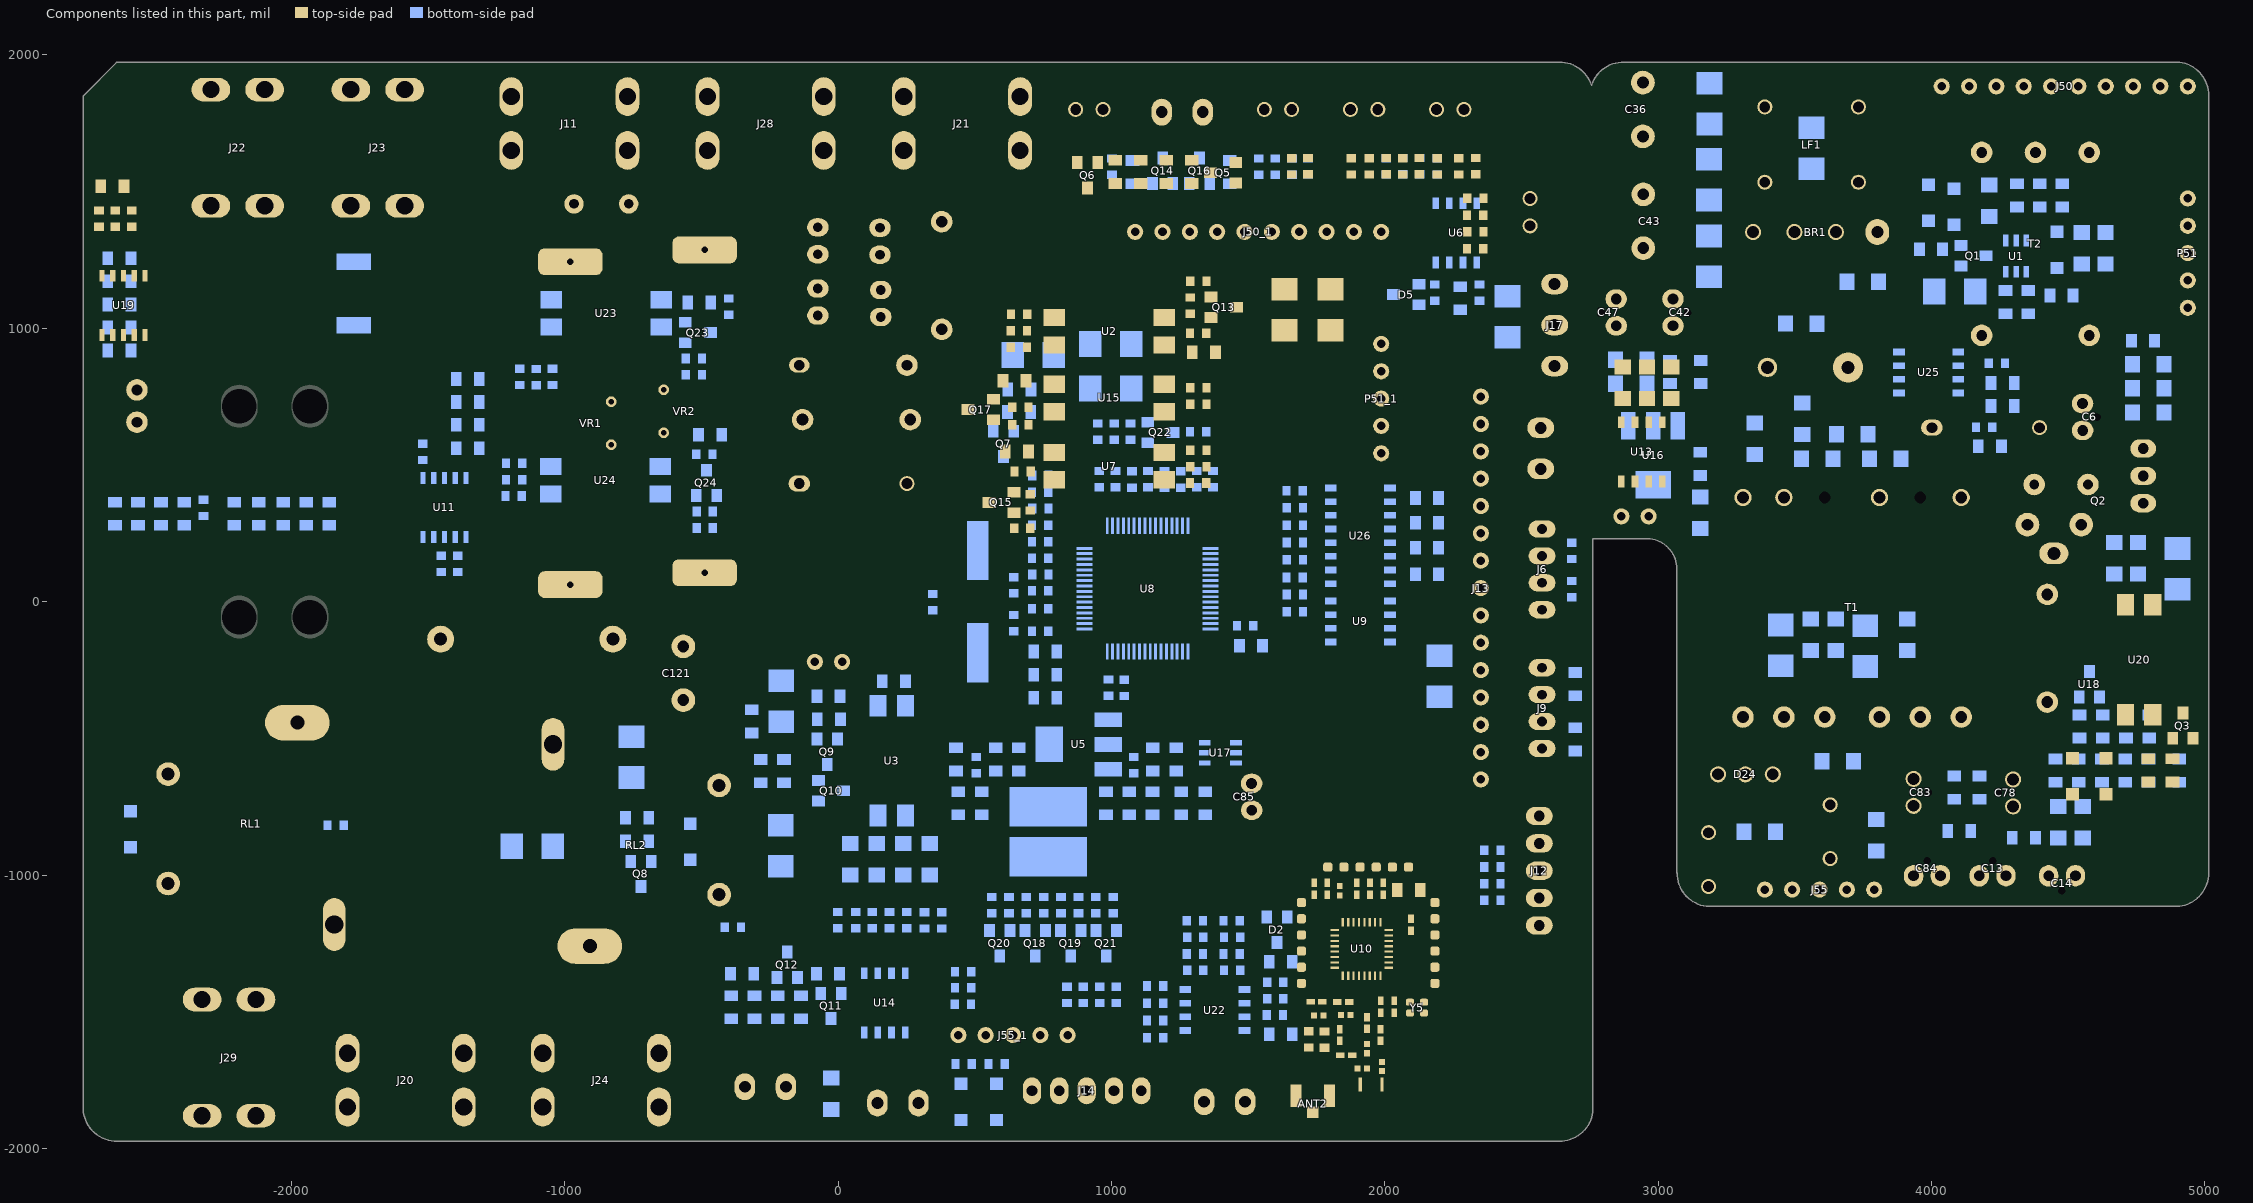
[diagram p0: the components of this part, seen from the top]
# Altium PCB MISC105418.PcbDoc (part 2 of 7)
Units mil, origin at the board's own origin, x right, y up, seen from the top; angles counter-clockwise.
Board outline 7774.32 x 3947.04 mil, 4 copper layers (Top Layer, 02, 03, Bottom Layer), stack 30.635 mil thick; 459 components, 285 nets, 1258 pads, 468 vias.
Unrouted connection lines stored in the file: 23.

## Components (designator, comment, footprint, x,y, rotation, side; value= is the part's Value field where it differs from the comment) (continued)
R38 "390K" R1206-T 2870,800 r270 top
R39 "390K" R1206-T 3048,800 r90 top
R40 "100R" R0603-T 661.16,930.81 r180 top
R41 "5.1K" R0603-T 950.04,622 r90 bottom
R42 "0R" R0402-T 1758.55,-1513.58 r0 top
R43 "1K" R0402-T 1835.09,-1057.41 r270 top
R44 "1M" R0603-T 346,-2 r90 bottom
R45 "2R" R1206-T 2901.87,884.55 r180 bottom
R46 "10K" R0603-T 1047,-315.46 r270 bottom
R47 "100R" R0603-T 752.1,-1109.77 r90 bottom
R48 "100R" R0603-T 879.04,-1109.77 r90 bottom
R49 "10K" R0603-T 688.63,-1109.77 r90 bottom
R50 "10K" R0603-T 815.57,-1109.77 r90 bottom
R51 "100R" R0603-T 625.16,-1109.77 r90 bottom
R52 "10K" R0603-T 561.69,-1109.77 r90 bottom
R53 "10K" R0603-T 1671.09,-37.5 r0 bottom
R54 "10K" R0603-T 1671.09,25.99 r0 bottom
R55 "10K" R0603-T 459.43,-1690.94 r180 bottom
R56 "1K" R0603-T 1539.09,1590.96 r270 bottom
R57 "1K" R0603-T 1002.09,1590.96 r90 bottom
R58 "10K" R0805-T 1432.09,1571.02 r270 bottom
R59 "10K" R0805-T 1077.09,1571.02 r270 bottom
R60 "100R" R0603-T -1.11,-1164.71 r90 bottom
R61 "4.7K" R0603-T 661.16,990.81 r180 top
R63 "470R" R0805-T 1338.05,911.91 r0 top
R64 "4.7K" R0603-T 1288.58,1083.07 r270 top
R65 "2K" R0603-T 1318.11,1171.91 r0 top
R66 "470R" R0805-T 653.68,549 r0 top
R67 "470R" R0805-T 663,776 r0 bottom
R68 "10K" R0805-T 662,694 r180 bottom
R69 "10K" R0805-T -35,-346 r180 bottom
R70 "5.1K" R0805-T -34,-430 r180 bottom
R71 "470R" R0805-T -735.12,-790.06 r0 bottom
R72 "470R" R0805-T -197.91,-620.12 r270 bottom
R73 "10K" R0805-T -282.91,-620.12 r270 bottom
R74 "10K" R0805-T -735.12,-876.15 r180 bottom
R75 "2K" R0805-T -37,-1360.82 r180 bottom
R77 "10K" R0603-T 457.21,-1353.53 r0 bottom
R78 "124K" R0603-T 64,-1164.71 r270 bottom
R79 "1.5K" R0603-T 457.21,-1412.5 r180 bottom
R80 "4.7K" R0603-T 703.15,363 r90 top
R81 "10K" R0603-T 188.3,-1164.71 r270 bottom
R82 "10K" R0603-T 251.44,-1164.71 r90 bottom
R83 "100R" RES/0603 1671.09,152.95 r0 bottom
R84 "10K" R0603-T 125.17,-1164.71 r270 bottom
R85 "2K" R0603-T 673.62,268 r0 top
R86 "4.7K" R0603-T 1318.11,493.41 r0 top
R87 "100R" R0603-T 1318.11,554 r180 top
R88 "2R" R1206-T 2901.87,796.5 r180 bottom
R89 "470R" R0805-T 645.06,808.3 r0 top
R90 "4.7K" R0603-T 667,711 r0 top
R91 "2K" R0603-T 667,647 r0 top
R92 "390K" R1206-T 2959,800 r90 top
R93 "100R" R0603-T 1318.11,722 r180 top
R94 "1.5M" R0805-T -1354.79,730.52 r180 bottom
R95 "1.2K" R1206-T 3154,324.52 r90 bottom
R96 "0R" R0805-T -2654.53,1519 r180 top
R97 "1K" R0805-T -135.91,-1483.82 r270 bottom
R99 "1K" R0805-T -220.91,-1483.82 r90 bottom
R100 "510K" R0805-T -390.91,-1483.82 r90 bottom
R102 "1.5M" R0805-T -1354.79,646.5 r0 bottom
R103 "10K" R0805-T -350.91,-1360.82 r0 bottom
R104 "4.7K" R0603-T -1044.5,822.48 r270 bottom
R105 "100R" R0603-T -1164.5,822.48 r270 bottom
R107 "470R" R0805-T -507.91,1094.5 r0 bottom
R108 "4.7K" R0603-T -527.85,889.5 r0 bottom
R109 "2K" R0603-T -527.85,829.5 r180 bottom
R110 "300R" R0805-T -467.91,610.76 r180 bottom
R111 "4.7K" R0603-T -487.85,329.5 r180 bottom
R112 "2K" R0603-T -487.85,269.5 r180 bottom
R113 "1K" R0603-T 2270,1592 r90 top
R114 "1K" R0603-T 2331.37,1476 r0 top
R115 "10K" R0603-T 1306.35,-1227.17 r180 bottom
R116 "1K" R0603-T 1075.04,446.82 r270 bottom
R117 "1K" R0603-T 1306.35,-1348.62 r180 bottom
R118 "10K" R0603-T 1440.91,-1227.17 r0 bottom
R119 "1K" R0603-T 1193.89,446.82 r270 bottom
R120 "1K" R0603-T 1440.91,-1348.62 r0 bottom
R121 "1K" R0603-T 1877,1592 r270 top
R122 "1K" R0603-T 1599.09,1590.96 r270 bottom
R123 "1.2K" R0805-T -1946.14,321.64 r270 bottom
R124 "1.2k" R0805-T -2209,321.64 r90 bottom
R125 "5.1K" R0603-T 837.45,-1438.62 r90 bottom
R126 "5.1K" R0603-T 1017.25,-1438.62 r90 bottom
R127 "100R" R0603-T 1005.98,-1109.77 r90 bottom
R128 "10K" R0603-T 942.51,-1109.77 r90 bottom
R129 "5.1K" R0805-T 1107.26,1572 r90 top
R130 "10K" R0805-T 1014.26,1572 r90 top
R133 "4.7K" R0603-T -1185.52,446.23 r180 bottom
R134 "100R" R0603-T -1185.52,506.5 r0 bottom
R135 "5.1K" R0805-T 1200.26,1572 r270 top
R136 "10K" R0805-T 1293.26,1572.02 r270 top
R137 "0R" R0603-T 2684.09,45.7 r90 bottom
R139 "0R" R0805-T 2696,-504 r270 bottom
R140 "0R" R0805-T 2696,-301.98 r90 bottom
R141 "NC" RES/0603 1671.09,343.4 r180 bottom
R142 "NC" RES/0603 1671.09,279.92 r180 bottom
R145 "1.2K" R0805-T -2119.69,321.64 r90 bottom
R147 "10K" R0603-T -2704,1400.76 r90 top
R148 "2.4M" R1206-T 3582.09,523.35 r180 bottom
R149 "2.4M" R1206-T 3710,612 r180 bottom
R150 "10K" R0603-T 2191.62,1592 r270 bottom
R151 "1K" R0603-T 1253.32,446.82 r270 bottom
R152 "10K" R0603-T 2331.37,1353.42 r0 top
R153 "1K" R0603-T 739.98,340.69 r0 bottom
R154 "10K" R0603-T 2004.81,1592 r270 bottom
R155 "1K" R0603-T 739.98,461.54 r0 bottom
R156 "NC" R0603-T 1943,1592 r90 top
R157 "1K" R0603-T 1659.85,1591.96 r270 top
R158 "1K" R0603-T 739.98,98.97 r0 bottom
R159 "NC" R0603-T 1660.28,1590.96 r90 bottom
R162 "10K" R0603-T -1451.91,138.5 r270 bottom
R163 "4.7K" R0603-T 1318.11,781.91 r0 top
R170 "0R" R0603-T 2684.09,185.98 r270 bottom
R171 "10K" R0603-T 1599.04,-1452.14 r0 bottom
R173 "10K" R0603-T 1159.25,-1532.29 r0 bottom
R174 "100R" R0603-T 1159.25,-1595.63 r0 bottom
R175 "100R" R0603-T 1159.25,-1468.96 r0 bottom
R176 "120R" R0805-T 1618.98,-1317.14 r0 bottom
R177 "100R" R0603-T 1159.25,-1405.63 r0 bottom
R178 "10K" R0603-T 1599.04,-1392.14 r180 bottom
R179 "120R" R0805-T 2276.09,1109.65 r90 bottom
R180 "100R" R0603-T 2065,1592 r90 top
R181 "100R" R0603-T 2192,1592 r270 top
R182 "1k" R0805-T -2476.66,321.64 r90 bottom
R183 "1mΩ" R2512-T -1772,1127 r270 bottom
R184 "1k" R0805-T -2645.15,321.64 r90 bottom
R185 "1.5M" R0805-T -2629.23,1255.67 r180 bottom
R186 "1.5M" R0805-T -2629.23,1171.42 r0 bottom
R187 "1.5M" R0805-T -2629.23,918.67 r180 bottom
R188 "1k" R0805-T -2629.23,1087.17 r180 bottom
R189 "10K" R0603-T -2584,1400.76 r270 top
R190 "10K" R0603-T -2644,1400.76 r270 top
R191 "2.4M" R1206-T 3831,523.35 r180 bottom
R192 "22K" R0805-T 4212.9,568.5 r180 bottom
R193 "1K" R0805-T 4259.9,799.53 r0 bottom
R194 "20K" R0805-T 4259.9,715.53 r180 bottom
R195 "30K" R1206-T 335.09,-943 r90 bottom
R196 "10K" R0805-T 204,-291 r0 bottom
R197 "1K" R0805-T 757.68,-267 r180 bottom
R198 "30K" R1206-T 141.76,-943 r270 bottom
R199 "2K" R0805-T 757.68,-351 r180 bottom
R200 "30K" R1206-T 45.09,-943 r90 bottom
R201 "2.4M" R1206-T 3526.98,669 r90 bottom
R213 "5.1K" R0603-T 897.25,-1438.34 r90 bottom
R214 "5.1K" R0603-T 957.25,-1438.62 r90 bottom
R231 "1.5M" R0805-T -1354.79,814.53 r0 bottom
R232 "1k" R0805-T -1354.79,561.5 r0 bottom
R233 "10K" R0603-T 2393.37,-909.5 r180 bottom
R234 "100R" R0603-T 2393.37,-1092.5 r180 bottom
R235 "100R" R0603-T 2393.37,-1031.5 r180 bottom
R236 "100R" R0603-T 2393.37,-970.5 r180 bottom
R237 "3K" R0603-T 1316.72,621 r180 bottom
R238 "100R" R0603-T 1009.7,622 r90 bottom
R239 "10K" R0603-T 1069.36,622 r90 bottom
R240 "10K" R0603-T 579.98,-1690.94 r0 bottom
R241 "1.5R" R1206-T 4793,692 r180 bottom
R260 "0R" R0402-T 1989.09,-1700.54 r90 top
R261 "0R" R0402-T 1917.55,-1708.03 r180 top
R263 "30K" R1206-T 238.43,-943 r90 bottom
R264 "10K" R0603-T -1391.91,138.5 r90 bottom
RL1 "T9VV1K15-12S" 继电器（T9VV1K15-12S） -1900.09,-589.46 r270 top
RL2 "T9VV1K15-12S" 继电器（T9VV1K15-12S） -986,-1113.48 r90 top
RNTC1 "NTC" R0603-t -385,-1191 r180 bottom
RNTC2 "NTC" R0603-t -1838,-818 r0 bottom
T1 "PQ20/20" PQ2020 3709.09,-20.5 r0 top
T2 "EFD30" 变压器 4379.85,1308.65 r180 top
U1 "OB2365E" SOT-23-6-T 4309,1264 r180 bottom
U2 "BPC-1009" OPT-SMT(LTV-817S) 992,988.91 r180 top
U3 "TLP785" OPT-SMT(LTV-817S) 196.09,-581.5 r90 bottom
U5 "AMS1117-3V3" SOT-223-T 878.06,-522.5 r270 bottom
U6 "TJA1050" SO-8-T 2261.09,1349.23 r0 bottom
U7 "BPC-1009" OPT-SMT(LTV-817S) 992,496 r0 top
U8 "AT403ARC" so-64-t1 1132.09,47.5 r270 bottom
U9 "AT24C16M/TR" SO-8-t 1910.09,-72.42 r270 bottom
U10 "TLSR8251" "QFN32 5X5MM" 1915.09,-1270.5 r180 top
U11 "BL0942" SO-10-T（脚距1.0mm) -1439.91,344.5 r0 bottom
U12 "CTZ-LB-10" "23012-00041-10  电流互感器" -2062.94,715.45 r270 top
U13 "OB222*" SO-8-t 2940,548 r180 top
U14 "LM2904" so-8-t 170.09,-1467.5 r180 bottom
U15 "BPC-1009" OPT-SMT(LTV-817S) 992,745 r0 top
U16 "AMS1117-3V3" SOT-223-T 2981,534 r0 bottom
U17 "SM8102H" SOT-23-6-T 1398,-553 r270 bottom
U18 "TL431" "SOT-23((TL431)(A K R)-T" 4577.09,-302.5 r180 bottom
U19 "BL0942" SO-10-T（脚距1.0mm) -2614,1084 r0 top
U20 "LTV-817C" OPT-SMT(LTV-817S) 4759.09,-212.5 r90 top
U22 "RS485" SO-8-T 1377.8,-1493.96 r90 bottom
U23 "BPC-1009" OPT-SMT(LTV-817S) -848.52,1054.5 r180 bottom
U24 "BPC-1009" OPT-SMT(LTV-817S) -850.91,444.12 r180 bottom
U25 "LM293" so-8-t 3989.09,838.5 r270 bottom
U26 "MAX232" SO-16-T 1910.09,240.7 r270 bottom
VR1 "TFMOV10M250" 防雷单元TFMOV10M -704.02,1322.03 r270 top
VR2 "TFMOV10M250" 防雷单元TFMOV10M -763.98,26.97 r90 top
Y1 "25MHz" SMD晶振（HC-49） 510,0 r270 bottom
Y2 "2.2nF/400V" CY7.5X4.7_P10_AI-DS 379,1193 r0 top
Y3 "2.2nF/400V" CY7.5X4.7_P10_AI-DS 67,666 r90 top
Y5 "24MHz" "23047-00020-11 32M SMD晶振" 2117.58,-1484.89 r0 top
ZC1 "Discharge tube SE801H-L" "ZC 8X6.5  P:16.0mm" -1139,-137 r0 bottom
ZD1 "13V" SOD-123-T 3989.09,1459.45 r270 bottom
ZD2 "6.2V" SOD-123-T 4638.09,-638.55 r270 top
ZD3 "12V" SOD-123-T 4515.09,-638.55 r270 top
? "Comment" 蓝牙 1938.83,-1183.58 r270 top
? "Comment" p2-2.54 2965,312 r180 top

## Footprints (in the part's own frame and the unit in brackets; to place one, negate y for a bottom-side part, rotate by r counter-clockwise, add the part's x,y. Pads: shape width x height; smd on the part's side, far side on the other; paste and mask are expansions set on the pad)
"23012-00041-10  电流互感器" [mm]
  round 2 hole 1: 1(-1.5,-12.75) 2(1.5,-12.75)
  silkscreen extent -12.5,-14.8 12.5,12.5
"23047-00020-11 32M SMD晶振" [mm]
  rrect50% 0.75x0.65 smd: 1(-0.65,-0.5) 2(0.65,-0.5) 3(0.65,0.5) 4(-0.65,0.5)
  silkscreen extent -1.42,-1.8 1.35,1.15
"71453-00013-11 (5X8.3 P:2.5)" [mm]
  oval 1.7x2 / inner round 1.3 / far side oval 1.7x2 hole 0.9: 1(-1.25,0) 2(1.25,0)
  silkscreen extent -2.75,-2.75 2.75,2.75, body extent -2.5,-2.5 2.5,2.5, height 8.3
ATN [mm]
  rect 0.3x1.3 smd mask+0.102: 1(1.01,0) 2(-1.01,0)
  Top Layer region: -1.503,-4.177 3.523,-4.177 3.523,-4.703 -1.503,-4.703
  Top Layer region: 0.797,0.713 1.323,0.713 1.323,-4.703 0.797,-4.703
  Top Layer region: 12.923,-0.237 12.397,-0.237 12.397,-4.703 12.923,-4.703 12.923,-0.237
  Top Layer region: -1.503,0.713 -0.577,0.713 -0.577,-4.703 -1.503,-4.703
  Top Layer region: 6.023,-4.703 5.497,-4.703 5.497,-1.537 6.023,-1.537 6.023,-4.703
  Top Layer region: 10.197,-4.177 12.923,-4.177 12.923,-4.703 10.197,-4.703 10.197,-4.177
  Top Layer region: 10.723,-4.703 10.197,-4.703 10.197,-1.537 10.723,-1.537 10.723,-4.703
  Top Layer region: 7.697,-1.537 10.723,-1.537 10.723,-2.063 7.697,-2.063 7.697,-1.537
  Top Layer region: 2.997,-4.703 3.523,-4.703 3.523,-1.537 2.997,-1.537 2.997,-4.703
  Top Layer region: 2.997,-1.537 6.023,-1.537 6.023,-2.063 2.997,-2.063 2.997,-1.537
  Top Layer region: 5.497,-4.177 8.223,-4.177 8.223,-4.703 5.497,-4.703 5.497,-4.177
  Top Layer region: 8.223,-1.537 7.697,-1.537 7.697,-4.703 8.223,-4.703 8.223,-1.537
ATN-1 [mm]
  rect 1.1x1.1 smd: 1(-1.55,0)
  rect 2.1x1 smd: 2(0,1.55) 2(0,-1.55)
  silkscreen extent -2.4,-2.32 2,2.32
BD15.22X4.5(KBP206）RS-2 [mm]
  oval 2.2x2.4 hole 1.1: 1(-5.775,0)
  round 1.5 / inner oval 2.2x2.4 / far side oval 2.2x2.4 hole 1.1: 2(-1.925,0) 3(1.93,0) 4(5.775,0)
  silkscreen extent -7.6,-2.98 7.6,3.1
C0402-T [mm]
  rect 0.79x0.54 smd: 1(-0.545,0) 2(0.545,0)
  silkscreen extent -1.17,-0.5 1.17,0.5
C0603-T [mm]
  rect 0.77x0.9 smd: 1(-0.755,0) 2(0.755,0)
  silkscreen extent -1.4,-0.65 1.4,0.65, body extent -0.8,-0.4 0.8,0.4, height 0.8
C0805-T [mm]
  rect 1x1.27 smd: 1(-1.075,0) 2(1.075,0)
  silkscreen extent -1.9,-0.95 1.9,0.96, body extent -1,-0.63 1,0.63, height 0.85
C1206-T [mm]
  rect 1.4x1.524 smd: 1(-1.462,0)
  rect 1.4x1.5 smd: 2(1.462,0)
  silkscreen extent -2.4,-1 2.4,1, body extent -1.6,-0.8 1.6,0.8, height 0.85
CAP/0603 [mm]
  rect 0.77x0.9 smd: 1(-0.755,0) 2(0.755,0)
  silkscreen extent -1.4,-0.65 1.4,0.65, body extent -0.8,-0.4 0.8,0.4, height 0.8
CAP/0805 [mm]
  rect 1x1.27 smd: 1(-1.075,0) 2(1.075,0)
  silkscreen extent -1.9,-0.95 1.9,0.96, body extent -1,-0.63 1,0.63, height 0.85
CC7.5-P5.0MM-AI-2.5-DS [mm]
  round 2.2 / inner round 1.5 / far side round 2.2 hole 1.1: 1(-2.5,0) 2(2.5,0)
  silkscreen extent -3.8,-1.24 3.7,1.26, body extent -4,-1.4 4,1.35, height 10
CE5-P2.5MM-AI [mm]
  round 0 hole 0.7 unplated: 0(0.01,1.38)
  oval 1.8x2 hole 1: 1(-1.245,-0.005) 2(1.245,0.005)
  silkscreen extent -2.54,-2.56 2.86,2.55, body extent -2.75,-2.75 2.75,2.75, height 12.8
CE5-P2.5MM-AI-DS [mm]
  round 0 hole 0.7 unplated: 0(0.01,1.38)
  oval 1.8x2 hole 1: 1(-1.245,-0.005) 2(1.245,0.005)
  silkscreen extent -2.54,-2.56 2.86,2.55, body extent -2.75,-2.75 2.75,2.75, height 12.8
CE6.3-P2.5MM-AI-DS [mm]
  round 0 hole 0.7 unplated: 0(0.01,1.38)
  oval 1.8x2 hole 1: 1(-1.245,-0.005) 2(1.245,0.005)
  silkscreen extent -3.2,-3.2 3.51,3.21, body extent -3.4,-3.4 3.4,3.4, height 12.8
CE8-P2.5MM-AI-DS [mm]
  round 0 hole 0.7 unplated: 0(0.015,1.398)
  round 1.5 / inner round 1.5 / far side oval 1.8x2.2 hole 1.1: 1(-1.25,0.023) 2(1.25,0.023)
  silkscreen extent -4.05,-4.04 4.54,4.06, body extent -4.25,-4.22 4.25,4.28, height 15
CE10-P5.0MM-AI [mm]
  round 0 hole 0.7 unplated: 0(-0.02,1.245)
  round 2.2 hole 1.1: 1(-2.51,0.035) 2(2.49,0.035)
  silkscreen extent -5.06,-5.07 5.42,5.08, body extent -5.26,-5.23 5.24,5.26, height 15
CE10-P5.0MM-AI-DS [mm]
  round 0 hole 0.7 unplated: 0(-0.02,1.245)
  round 2.2 hole 1.1: 1(-2.51,0.035) 2(2.49,0.035)
  silkscreen extent -5.06,-5.07 5.42,5.08, body extent -5.26,-5.23 5.24,5.26, height 15
CE18 [mm]
  round 2.8 hole 1.2: 1(-3.75,0)
  round 1.8 / inner round 1.8 / far side round 2.8 hole 1.2: 2(3.75,0)
  silkscreen extent -9.05,-9.05 9.61,9.05, body extent -9.25,-9.25 9.25,9.25, height 25
CON2-2.54 [mm]
  round 1.4 / inner round 1.4 / far side oval 1.7x2.5 hole 1: 1(-1.27,0) 2(1.27,0)
  silkscreen extent -3.77,-4.01 3.91,2, body extent -3.85,-4.13 4.03,2.1, height 7.5
con2-2.54 [mm]
  round 1.4 / inner round 1.4 / far side oval 1.7x2.5 hole 1: 1(-1.27,0) 2(1.27,0)
  silkscreen extent -3.77,-4.01 3.91,2, body extent -3.85,-4.13 4.03,2.1, height 7.5
CON2-3.81 [mm]
  oval 1.9x2.5 hole 1.1: 1(-1.905,0) 2(1.905,0)
  silkscreen extent -4.62,-3 4.68,4.33, body extent -4.61,-3.02 4.64,4.34, height 9.2
CON3-3.81 [mm]
  oval 1.9x2.5 hole 1.1: 1(-3.81,0) 2(0,0) 3(3.81,0)
  silkscreen extent -6.53,-3 6.56,4.33, body extent -6.52,-3.02 2.74,4.34, height 9.2
CON4-2.5 [mm]
  oval 1.6x2.5 hole 0.9: 1(-3.75,0) 2(-1.25,0) 3(1.25,0) 4(3.75,0)
  silkscreen extent -6.25,-2.3 6.2,4.19, body extent -6.35,-2.43 6.3,4.3, height 7.5
CON5-2.54 [mm]
  oval 1.7x2.5 hole 1: 1(-5.08,0) 2(-2.54,0) 3(0,0) 4(2.54,0) 5(5.08,0)
  silkscreen extent -7.58,-4.01 7.72,2, body extent -7.7,-4.1 7.85,2.13, height 7.5
CX10.0X4.0-P7.5 [mm]
  round 2 hole 1 mask+0.05: 1(-4.325,0)
  oval 1.9x1.4 / inner oval 1.9x1.4 / far side oval 2.7x2 hole 1 slot 1.5 at 0 deg mask+0.05: 2(5.675,0)
  silkscreen extent -5.42,-2.25 6.63,2.25, body extent -5.25,-2.25 5.25,2.25, height 15
CX12.0X6.0-P10 [mm]
  round 1.4 / inner round 1.4 / far side round 2 hole 1 mask+0.05: 1(-5,0)
  oval 2x1.5 / inner oval 2x1.5 / far side oval 2.7x2 hole 1 slot 1.5 at 0 deg mask+0.05: 2(5,0)
  silkscreen extent -5.91,-3.04 6.09,2.96, body extent -6.05,-3.18 6.22,3.1, height 15
CY7.5X4.7_P10_AI-DS [mm]
  round 2 / inner round 1.5 / far side round 2 hole 1.1: 1(0,-5) 2(0,5)
  silkscreen extent -2.64,-4.85 2.64,4.92, body extent -2.64,-5.58 2.66,5.52, height 15
FUSE-TE5 [mm]
  round 1.8 hole 0.9: 1(-2.54,0) 2(2.54,0)
  silkscreen extent -4.29,-2 4.21,2, body extent -4.3,-2 4.2,2, height 7.8
L(8x8x4)-3d [mm]
  rect 3.65x7.2 smd: 1(-2.325,0) 2(2.325,0)
  silkscreen extent -4.5,-3.9 4.5,3.9, body extent -3.68,-3.75 3.75,3.76, height 5
L-DR6-P5.0 [mm]
  round 1.4 / inner round 1.4 / far side round 2.2 hole 1: 1(-2.5,0) 2(2.5,0)
  silkscreen extent -3.05,-3.05 3.05,3.05
OPT-SMT(LTV-817S) [mm]
  rect 2x1.6 smd: 1(-5.1,1.27) 2(-5.1,-1.27) 3(5.1,-1.27) 4(5.1,1.27)
  silkscreen extent -6.57,-2.55 6.57,3.29, body extent -5.1,-2.55 5.1,2.55, height 4.6
p2-2.54 [mm]
  round 1.5 hole 0.8: 1(0,0) 2(2.54,0)
  silkscreen extent -1.27,-1.27 3.81,1.27
P5-2.54 [mm]
  round 1.5 hole 0.8: 1(0,0) 2(2.54,0) 3(5.08,0) 4(7.62,0) 5(10.16,0)
  silkscreen extent -1.27,-1.27 11.43,1.27
p10-2.54 [mm]
  round 1.5 hole 0.8: 1(0,0) 2(2.54,0) 3(5.08,0) 4(7.62,0) 5(10.16,0) 6(12.7,0) 7(15.24,0) 8(17.78,0) 9(20.32,0) 10(22.86,0)
  silkscreen extent -1.27,-1.27 24.13,1.27
P15-2.54 [mm]
  round 1.5 hole 0.8: 1(0,0) 2(0,-2.54) 3(0,-5.08) 4(0,-7.62) 5(0,-10.16) 6(0,-12.7) 7(0,-15.24) 8(0,-17.78) 9(0,-20.32) 10(0,-22.86) 11(0,-25.4) 12(0,-27.94) 13(0,-30.48) 14(0,-33.02) 15(0,-35.56)
  silkscreen extent -1.27,-36.83 1.27,1.27
PQ2020 [mm]
  round 1.6 / inner round 1.5 / far side round 2.5 hole 1.1: 1(10.14,10.2) 3(2.54,10.2) 5(-6.34,10.2) 6(-10.14,10.2)
  round 0 hole 1.1: 2(6.34,10.2) 4(-2.54,10.2)
  round 2 hole 1.1: 7(-10.14,-10.2) 8(-6.34,-10.2) 9(-2.54,-10.2) 10(2.54,-10.2) 11(6.34,-10.2) 12(10.14,-10.2)
  silkscreen extent -12,-13 12,13
"QFN32 5X5MM" [mm]
  rect 0.8x0.2 smd: 1(-2.5,1.75) 2(-2.5,1.25) 3(-2.5,0.75) 4(-2.5,0.25) 5(-2.5,-0.25) 6(-2.5,-0.75) 7(-2.5,-1.25) 8(-2.5,-1.75) 17(2.5,-1.75) 18(2.5,-1.25) 19(2.5,-0.75) 20(2.5,-0.25) 21(2.5,0.25) 22(2.5,0.75) 23(2.5,1.25) 24(2.5,1.75)
  rect 0.2x0.8 smd: 9(-1.75,-2.5) 10(-1.25,-2.5) 11(-0.75,-2.5) 12(-0.25,-2.5) 13(0.25,-2.5) 14(0.75,-2.5) 15(1.25,-2.5) 16(1.75,-2.5) 25(1.75,2.5) 26(1.25,2.5) 27(0.75,2.5) 28(0.25,2.5) 29(-0.25,2.5) 30(-0.75,2.5) 31(-1.25,2.5) 32(-1.75,2.5)
  silkscreen extent -2.9,-2.9 2.9,2.9
R0402-T [mm]
  rect 0.566x0.54 smd: 1(-0.433,0) 2(0.433,0)
  silkscreen extent -0.94,-0.5 0.94,0.5
R0603-T [mm]
  rect 0.77x0.9 smd: 1(-0.755,0) 2(0.755,0)
  silkscreen extent -1.43,-0.68 1.43,0.68, body extent -0.8,-0.4 0.8,0.4, height 0.45
R0603-t [mm]
  rect 0.77x0.9 smd: 1(-0.755,0) 2(0.755,0)
  silkscreen extent -1.43,-0.68 1.43,0.68, body extent -0.8,-0.4 0.8,0.4, height 0.45
R0805-T [mm]
  rect 1x1.27 smd: 1(-1.075,0) 2(1.075,0)
  silkscreen extent -1.9,-0.95 1.9,0.95, body extent -1,-0.63 1,0.63, height 0.5
R1206-T [mm]
  rect 1.4x1.525 smd: 1(-1.462,0) 2(1.462,0)
  silkscreen extent -2.4,-1 2.4,1, body extent -1.55,-0.8 1.55,0.8, height 0.55
R2512-T [mm]
  rect 1.5x3.2 smd: 1(-2.95,0) 2(2.95,0)
  silkscreen extent -4,-1.9 4,1.9, body extent -3.18,-1.6 3.17,1.6, height 0.55
R-1W-P5.0-V [mm]
  round 2 / inner round 1.3 / far side round 2 hole 0.9: 1(-2.5,0) 2(2.5,0)
  silkscreen extent -4.5,-2 2,2
RES/0603 [mm]
  rect 0.77x0.9 smd: 1(-0.755,0) 2(0.755,0)
  silkscreen extent -1.43,-0.68 1.43,0.68, body extent -0.8,-0.4 0.8,0.4, height 0.45
SMA [mm]
  rect 2.1x2.4 smd: 1(-1.9,0) 2(1.9,0)
  silkscreen extent -3.4,-1.52 3.46,2.46, body extent -2.3,-1.35 2.3,1.35, height 2.4
SMA-T [mm]
  rect 2.1x2.4 smd: 1(-1.9,0) 2(1.9,0)
  silkscreen extent -3.4,-1.52 3.46,2.46, body extent -2.3,-1.35 2.3,1.35, height 2.4
SMD晶振（HC-49） [mm]
  rect 5.5x2 smd: 1(-4.75,0) 2(4.75,0)
  silkscreen extent -5.75,-2.5 5.75,2.5, body extent -6.95,-2.5 6.95,2.5, height 4.1
SO-8-T [mm]
  rect 0.62x1.1 smd: 1(-1.905,-2.75) 2(-0.635,-2.75) 3(0.635,-2.75) 4(1.905,-2.75) 5(1.905,2.75) 6(0.635,2.75) 7(-0.635,2.75) 8(-1.905,2.75)
  silkscreen extent -2.85,-3.35 2.61,3.35, body extent -2.45,-3 2.45,3, height 1.55
SO-8-t [mm]
  rect 0.62x1.1 smd: 1(-1.905,-2.75) 2(-0.635,-2.75) 3(0.635,-2.75) 4(1.905,-2.75) 5(1.905,2.75) 6(0.635,2.75) 7(-0.635,2.75) 8(-1.905,2.75)
  silkscreen extent -2.85,-3.35 2.61,3.35, body extent -2.45,-3 2.45,3, height 1.55
so-8-t [mm]
  rect 0.62x1.1 smd: 1(-1.905,-2.75) 2(-0.635,-2.75) 3(0.635,-2.75) 4(1.905,-2.75) 5(1.905,2.75) 6(0.635,2.75) 7(-0.635,2.75) 8(-1.905,2.75)
  silkscreen extent -2.85,-3.35 2.61,3.35, body extent -2.45,-3 2.45,3, height 1.55
SO-10-T（脚距1.0mm) [mm]
  rect 0.5x1.1 smd: 1(-2,-2.75) 2(-1,-2.75) 3(0,-2.75) 4(1,-2.75) 5(2,-2.75) 6(2,2.75) 7(1,2.75) 8(0,2.75) 9(-1,2.75) 10(-2,2.75)
  silkscreen extent -3.49,-3.4 2.55,3.35, body extent -2.55,-2.95 2.55,2.95, height 1.75
SO-16-T [mm]
  rect 0.62x1.1 smd: 1(-4.445,-2.75) 2(-3.175,-2.75) 3(-1.905,-2.75) 4(-0.635,-2.75) 5(0.635,-2.75) 6(1.905,-2.75) 7(3.175,-2.75) 8(4.445,-2.75) 9(4.445,2.75) 10(3.175,2.75) 11(1.905,2.75) 12(0.635,2.75) 13(-0.635,2.75) 14(-1.905,2.75) 15(-3.175,2.75) 16(-4.445,2.75)
  silkscreen extent -5.39,-3.35 5.15,3.35, body extent -4.99,-3 4.99,3, height 1.55
so-64-t1 [mm]
  rect 0.27x1.5 smd: 1(3.75,5.85) 2(3.25,5.85) 3(2.75,5.85) 4(2.25,5.85) 5(1.75,5.85) 6(1.25,5.85) 7(0.75,5.85) 8(0.25,5.85) 9(-0.25,5.85) 10(-0.75,5.85) 11(-1.25,5.85) 12(-1.75,5.85) 13(-2.25,5.85) 14(-2.75,5.85) 15(-3.25,5.85) 16(-3.75,5.85) 33(-3.75,-5.85) 34(-3.25,-5.85) 35(-2.75,-5.85) 36(-2.25,-5.85) 37(-1.75,-5.85) 38(-1.25,-5.85) 39(-0.75,-5.85) 40(-0.25,-5.85) 41(0.25,-5.85) 42(0.75,-5.85) 43(1.25,-5.85) 44(1.75,-5.85) 45(2.25,-5.85) 46(2.75,-5.85) 47(3.25,-5.85) 48(3.75,-5.85)
  rect 1.5x0.27 smd: 17(-5.85,3.75) 18(-5.85,3.25) 19(-5.85,2.75) 20(-5.85,2.25) 21(-5.85,1.75) 22(-5.85,1.25) 23(-5.85,0.75) 24(-5.85,0.25) 25(-5.85,-0.25) 26(-5.85,-0.75) 27(-5.85,-1.25) 28(-5.85,-1.75) 29(-5.85,-2.25) 30(-5.85,-2.75) 31(-5.85,-3.25) 32(-5.85,-3.75) 49(5.85,-3.75) 50(5.85,-3.25) 51(5.85,-2.75) 52(5.85,-2.25) 53(5.85,-1.75) 54(5.85,-1.25) 55(5.85,-0.75) 56(5.85,-0.25) 57(5.85,0.25) 58(5.85,0.75) 59(5.85,1.25) 60(5.85,1.75) 61(5.85,2.25) 62(5.85,2.75) 63(5.85,3.25) 64(5.85,3.75)
  silkscreen extent -4.65,-4.66 4.7,4.7
SOD-123-T [mm]
  rect 1.15x1.2 smd: 1(-1.675,0) 2(1.675,0)
  silkscreen extent -2.6,-1.1 2.98,1.97, body extent -1.85,-0.8 1.85,0.8, height 1.2
"SOT-23((TL431)(A K R)-T" [mm]
  rect 1x1.2 smd: A(0,1.175) K(0.95,-1.175) R(-0.95,-1.175)
  silkscreen extent -1.5,-0.39 1.5,0.42, body extent -1.45,-1.2 1.45,1.2, height 1
SOT-23-6-T [mm]
  rect 0.5x1.1 smd: 1(-0.95,-1.46) 2(0,-1.46) 3(0.95,-1.46) 4(0.95,1.45) 5(0,1.45) 6(-0.95,1.45)
  silkscreen extent -1.51,-1.54 1.5,0.8, body extent -1.45,-1.4 1.45,1.4, height 1.45
SOT-23-T [mm]
  rect 1x1.2 smd: 1(-0.95,-1.175) 2(0.95,-1.175) 3(0,1.175)
  silkscreen extent -1.5,-0.39 1.5,0.42, body extent -1.45,-1.2 1.45,1.2, height 1
SOT-223-T [mm]
  rect 1.35x2.55 smd: 1(-2.31,-2.795) 2(0,-2.795) 3(2.31,-2.795)
  rect 3.3x2.55 smd: 2(0,2.685)
  silkscreen extent -3.32,-4.4 3.32,1.29, body extent -3.33,-3.34 3.32,3.28, height 1
"TO-220((散热片16.5X16mm 厚1.5mm)" [mm]
  oval 2x2.7 hole 1.2 slot 1.5 at 90 deg: 0(9.74,-8.3)
  oval 1.7x2.4 hole 1: 1(0,0) 2(2.54,0) 3(5.08,0)
  silkscreen extent -4.86,-11.7 11.64,4.51, body extent -4.86,-11.7 11.64,4.5, height 22.5
TO-220(AKA二极管） [mm]
  round 1.5 / inner round 1.5 / far side oval 1.8x2.4 hole 1.1: 1(-2.54,0) 2(0,0) 3(2.54,0)
  silkscreen extent -5.3,-1.64 5.3,3, body extent -5.1,-1.8 5.1,2.7, height 19.5
"UU9.8 - (8.7MM)" [mm]
  round 1.4 / inner round 1.4 / far side round 2.2 hole 1: 1(-4.35,-3.5) 2(-4.35,3.5) 3(4.35,-3.5) 4(4.35,3.5)
  silkscreen extent -7.9,-6.27 7.9,6.26
"ZC 8X6.5  P:16.0mm" [mm]
  round 2.5 hole 1.2: 1(-8,0)
  round 1.6 / inner round 1.6 / far side round 2.5 hole 1.2: 2(8,0)
  silkscreen extent -7.5,-4 7.5,4
变压器 [mm]
  round 2 hole 1: 1(-5,-8.5) 2(5,-8.5) 3(-5,8.5) 4(5,8.5) 5(0,-8.5)
  silkscreen extent -12,-12.85 12,12.85
接线端子（12X9mm） [mm]
  oval 2.2x3.6 / inner oval 3.5x5 / far side oval 3.5x5 hole 1.6 slot 3 at 90 deg: 1(-5.4,-2.5) 1(-5.4,2.5) 1(5.4,-2.5) 1(5.4,2.5)
  silkscreen extent -7.5,-5.25 7.5,5.25
继电器（T9VV1K15-12S） [mm]
  oval 3.3x6 hole 1.3 slot 3.8 at 90 deg: 1(-3.725,-1.98)
  round 2.2 hole 1.2: 2(1.055,-13.99) 3(11.215,-13.99)
  oval 4.9x2.1 / inner oval 4.9x2.1 / far side oval 6.8x4 hole 1.7 slot 4.5 at 0 deg: 4(15.025,1.45)
  silkscreen extent -7.1,-21.15 20.41,11.45, body extent -7.1,-21.15 20.4,11.45, height 20.4
蓝牙 [mm]
  rrect50% 0.85x0.85 smd: 12(-5.401,2.25) 12(-5.401,3.75) 12(-5.401,-0.75) 12(-5.401,0.75) 12(-5.401,-3.75) 12(-5.401,-2.25) 12(-2.099,6.202) 12(-2.099,-6.202) 12(-0.599,6.202) 12(-0.599,-6.202) 12(0.901,6.202) 12(0.901,-6.202) 12(2.401,6.202) 12(2.401,-6.202) 12(3.901,6.202) 12(3.901,-6.202) 12(5.401,6.202) 12(5.401,-6.202)
  silkscreen extent -5.4,-6.2 20.23,6.2
防雷单元TFMOV10M [mm]
  rrect50% 2.5x6 hole 0.6 slot 5 at 90 deg: 1(32,-7) 2(2,-7)
  round 1 hole 0.5: 3(19,-3.2) 4(15,-3.2)
  silkscreen extent 0,-14.08 34,0